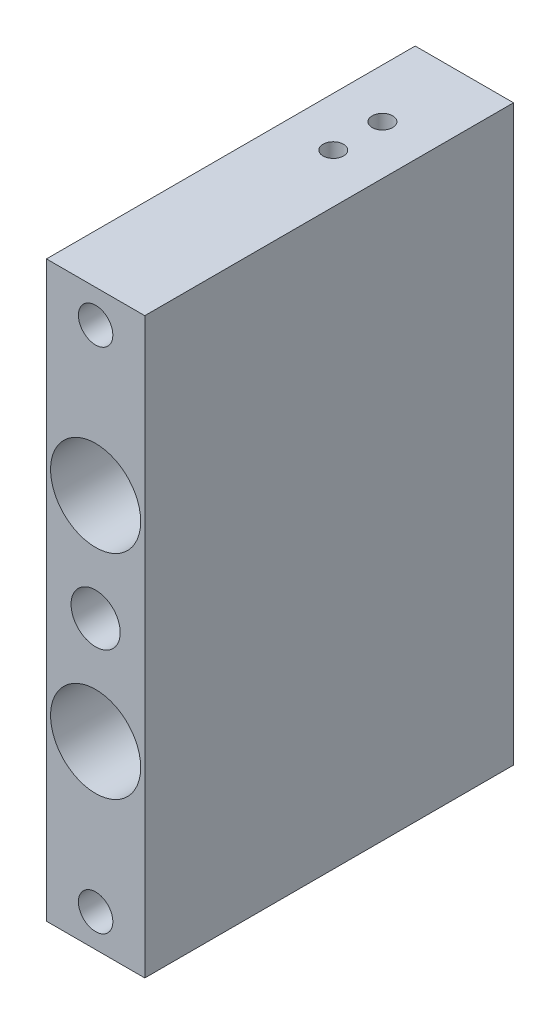
from build123d import *

# Parameters (mm, degrees)
SKETCH_13_W               = 12
SKETCH_13_H               = 70
EXTRUDE_1_DEPTH           = 45
HOLE_WIZARD_M3_1_D        = 2.5
HOLE_WIZARD_M3_1_DEPTH    = 12.5
HOLE_WIZARD_M3_1_TIP      = 0.751075774
HOLE_WIZARD_M5_1_D        = 4.2
HOLE_WIZARD_M5_1_DEPTH    = 19
HOLE_WIZARD_M5_1_TIP      = 1.2618073
HOLE_WIZARD_1_D           = 6.4
HOLE_WIZARD_1_CBORE_D     = 11
HOLE_WIZARD_1_CBORE_DEPTH = 20
HOLE_WIZARD_6_0_6_1_D     = 6
HOLE_WIZARD_6_0_6_1_DEPTH = 10
HOLE_WIZARD_6_0_6_1_TIP   = 1.802581857
HOLE_WIZARD_6_0_6_2_D     = 6
HOLE_WIZARD_6_0_6_2_DEPTH = 10
HOLE_WIZARD_6_0_6_2_TIP   = 1.802581857


with BuildPart() as part:
    # 草图13 → 凸台-拉伸1 (new body)
    with BuildSketch(Plane.XY):
        Rectangle(SKETCH_13_W, SKETCH_13_H)
    extrude(amount=EXTRUDE_1_DEPTH)

    # M3 螺纹孔1
    with Locations(Plane(origin=(0, 35, 0), x_dir=(1, 0, 0), z_dir=(0, 1, 0))):
        with Locations((0, -10), (0, -16)):
            Hole(HOLE_WIZARD_M3_1_D / 2, depth=HOLE_WIZARD_M3_1_DEPTH)
            with Locations((0, 0, -(HOLE_WIZARD_M3_1_DEPTH + HOLE_WIZARD_M3_1_TIP / 2))):  # 118° drill point
                Cone(0, HOLE_WIZARD_M3_1_D / 2, HOLE_WIZARD_M3_1_TIP, mode=Mode.SUBTRACT)

    # M5 螺纹孔1
    with Locations(Plane.XY.offset(45)):
        with Locations((0, 31), (0, -31)):
            Hole(HOLE_WIZARD_M5_1_D / 2, depth=HOLE_WIZARD_M5_1_DEPTH)
            with Locations((0, 0, -(HOLE_WIZARD_M5_1_DEPTH + HOLE_WIZARD_M5_1_TIP / 2))):  # 118° drill point
                Cone(0, HOLE_WIZARD_M5_1_D / 2, HOLE_WIZARD_M5_1_TIP, mode=Mode.SUBTRACT)

    # 打孔尺寸(%根据)内六角圆柱头螺钉的类型1 (through all)
    with Locations(Plane.XY.offset(45)):
        with Locations((0, 13), (0, -13)):
            CounterBoreHole(HOLE_WIZARD_1_D / 2, HOLE_WIZARD_1_CBORE_D / 2, HOLE_WIZARD_1_CBORE_DEPTH)

    # Ø6.0 (6) 直径孔1
    with Locations(Plane.XY.offset(45)):
        with Locations((0, 0)):
            Hole(HOLE_WIZARD_6_0_6_1_D / 2, depth=HOLE_WIZARD_6_0_6_1_DEPTH)
            with Locations((0, 0, -(HOLE_WIZARD_6_0_6_1_DEPTH + HOLE_WIZARD_6_0_6_1_TIP / 2))):  # 118° drill point
                Cone(0, HOLE_WIZARD_6_0_6_1_D / 2, HOLE_WIZARD_6_0_6_1_TIP, mode=Mode.SUBTRACT)

    # Ø6.0 (6) 直径孔2
    with Locations(Plane(origin=(0, 0, 0), x_dir=(-1, 0, 0), z_dir=(0, 0, -1))):
        with Locations((0, -22.5), (0, 22.5)):
            Hole(HOLE_WIZARD_6_0_6_2_D / 2, depth=HOLE_WIZARD_6_0_6_2_DEPTH)
            with Locations((0, 0, -(HOLE_WIZARD_6_0_6_2_DEPTH + HOLE_WIZARD_6_0_6_2_TIP / 2))):  # 118° drill point
                Cone(0, HOLE_WIZARD_6_0_6_2_D / 2, HOLE_WIZARD_6_0_6_2_TIP, mode=Mode.SUBTRACT)


solid = part.part
